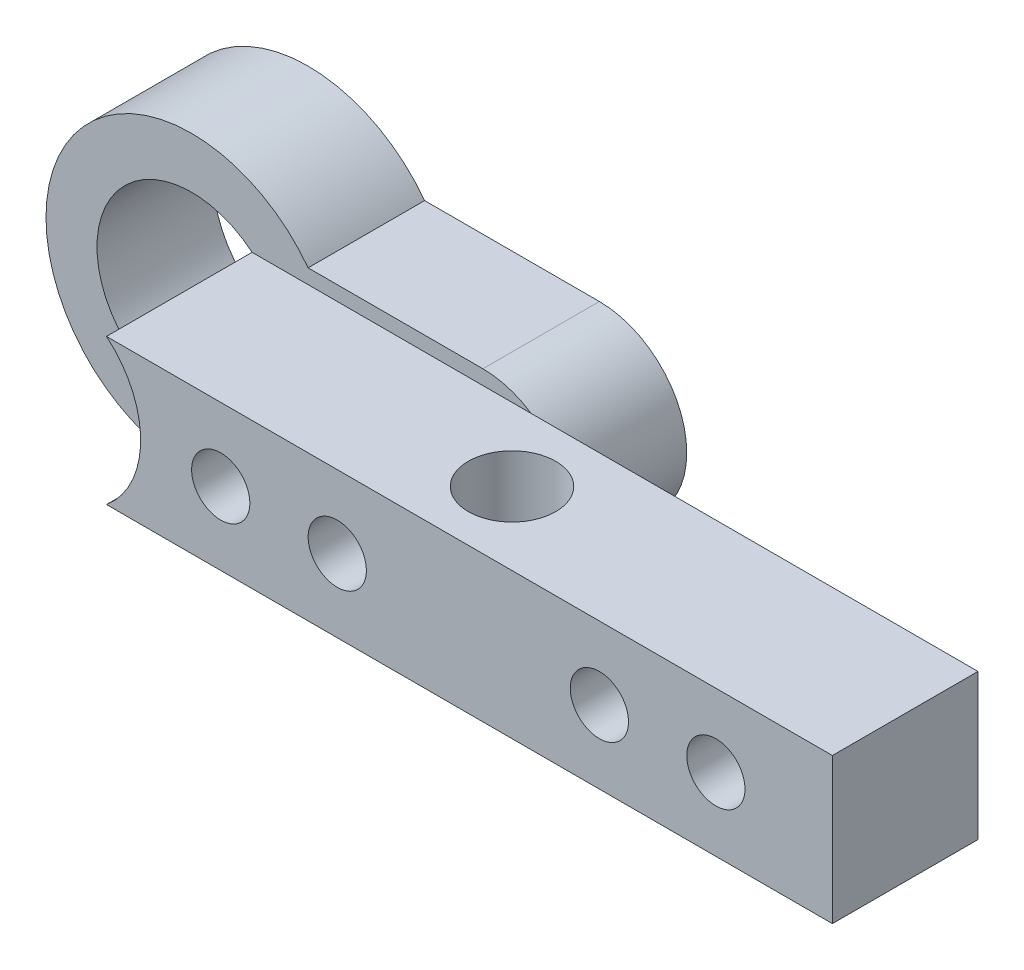
SolidWorks part; units mm, degrees
ref_plane "Front Plane" through (0, 0, 0) normal (0, 0, 1) x (1, 0, 0)
ref_plane "Top Plane" through (0, 0, 0) normal (0, 1, 0) x (1, 0, 0)
ref_plane "Right Plane" through (0, 0, 0) normal (1, 0, 0) x (0, 0, -1)
other "Configuration Table"
sketch "Sketch1" plane through (0, 0, 0) normal (0, 1, 0) x (1, 0, 0)
  line L0 (25, 0) -> (25, -10) construction
  line L1 (0, 0) -> (50, 0)
  line L2 (0, 0) -> (0, -10)
  line L3 (0, -10) -> (50, -10)
  line L4 (50, 0) -> (50, -10)
  dimension "D1" = 50
  dimension "D2" = 10
extrude "Boss-Extrude1" add sketch "Sketch1" along normal blind 10
sketch "Sketch2" plane through (0, 10, 0) normal (0, 1, 0) x (1, 0, 0)
  line L0 (25, 0) -> (25, -10) construction
  line L1 (50, 0) -> (0, 0) construction
  line L2 (0, -10) -> (50, -10) construction
  circle A0 centre (23, -5) radius 3
  dimension "D1" = 6
  dimension "D3" = 2
extrude "Cut-Extrude1" cut sketch "Sketch2" against normal blind 10
sketch "Sketch3" plane through (0, 0, 10) normal (0, 0, 1) x (1, 0, 0)
  line L0 (25, 10) -> (25, 0) construction
  line L1 (0, 10) -> (50, 10) construction
  line L2 (0, 0) -> (50, 0) construction
  circle A0 centre (8, 5) radius 2
  circle A1 centre (16, 5) radius 2
  circle A2 centre (42, 5) radius 2
  circle A3 centre (34, 5) radius 2
  dimension "D1" = 4
  dimension "D2" = 4
  dimension "D3" = 16
  dimension "D4" = 8
  dimension "D5" = 5
  dimension "D6" = 5
extrude "Cut-Extrude2" cut sketch "Sketch3" against normal blind 10
sketch "Sketch4" plane through (0, 0, 0) normal (0, 0, -1) x (-1, 0, 0)
  line L0 (-16, 11) -> (-4, 11)
  line L1 (-16, -1) -> (-4, -1)
  arc A0 (-16, 11) -> (-16, -1) centre (-16, 5) ccw
  arc A1 (-4, -1) -> (-4, 11) centre (4, 5) ccw
  dimension "D1" = 12
  dimension "D2" = 20
  dimension "D4" = 5
  dimension "D3" = 20
extrude "Boss-Extrude2" add sketch "Sketch4" along normal blind 30
sketch "Sketch5" plane through (0, 0, -30) normal (0, 0, -1) x (-1, 0, 0)
  circle A1 centre (4, 5) radius 6.5
  dimension "D2" = 13
sketch "Sketch6" plane through (0, -1, 0) normal (0, -1, 0) x (1, 0, 0)
  line L0 (16, 0) -> (4, 0) construction
  line L1 (27.6913, -33) -> (-19.3087, -33)
  line L2 (27.6913, -33) -> (27.6913, -8)
  line L3 (27.6913, -8) -> (-19.3087, -8)
  line L4 (-19.3087, -33) -> (-19.3087, -8)
  dimension "D1" = 8
  dimension "D2" = 25
  dimension "D3" = 47
extrude "Cut-Extrude4" cut sketch "Sketch6" against normal through all both and the other way through all
sketch "Sketch7" plane through (0, 0, 0) normal (0, 0, 1) x (1, 0, 0)
  circle A0 centre (8, 5) radius 2
  circle A1 centre (16, 5) radius 2
  dimension "D1" = 4
  dimension "D2" = 4
extrude "Cut-Extrude5" cut sketch "Sketch7" against normal through all both and the other way through all
extrude "Cut-Extrude6" cut sketch "Sketch5" against normal through all
